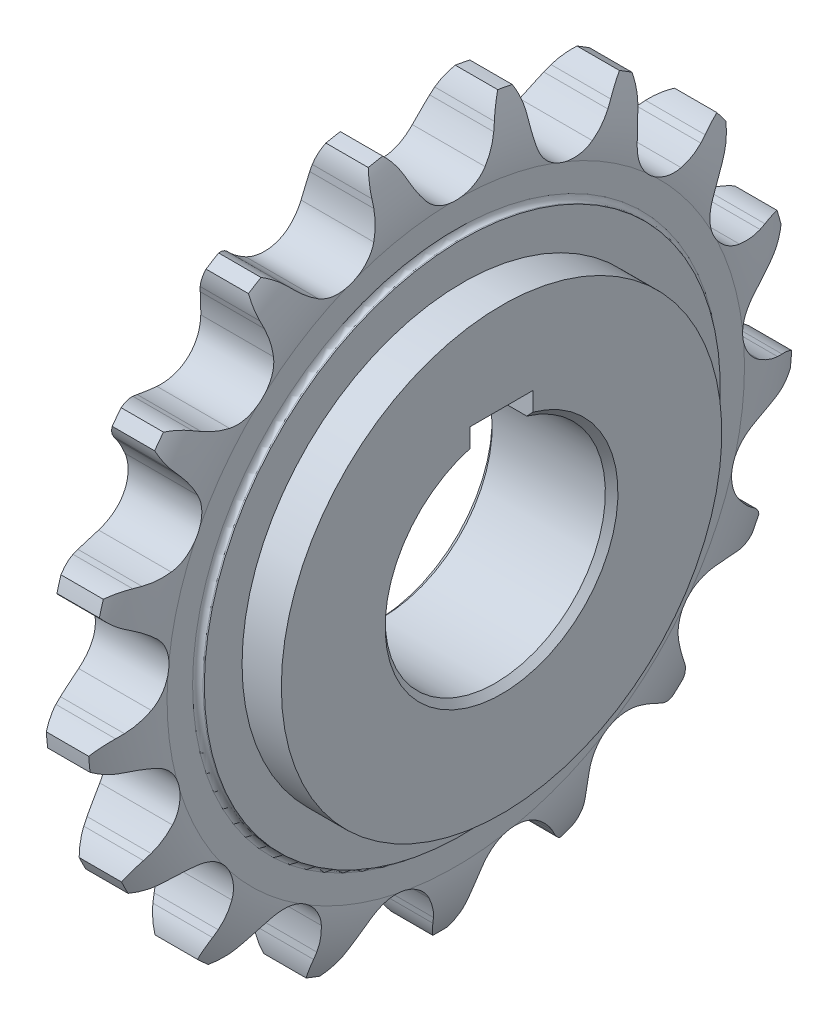
SolidWorks part; units mm, degrees
ref_plane "前视基准面" through (0, 0, 0) normal (0, 0, 1) x (1, 0, 0)
ref_plane "上视基准面" through (0, 0, 0) normal (0, 1, 0) x (1, 0, 0)
ref_plane "右视基准面" through (0, 0, 0) normal (1, 0, 0) x (0, 0, -1)
sketch "草图1" plane through (0, 0, 0) normal (0, 0, 1) x (1, 0, 0)
  line L0 (-9.525, 0) -> (9.525, 0) construction
  line L1 (-6.88, 17.5) -> (-6.88, 41)
  line L2 (-6.88, 41) -> (-6.673, 41)
  line L3 (-5.845, 41.8279) -> (-5.845, 45.8819)
  line L4 (-3.3685, 56) -> (3.3685, 56)
  line L5 (5.845, 45.8819) -> (5.845, 41.8279)
  line L6 (6.673, 41) -> (6.88, 41)
  line L7 (6.88, 41) -> (6.88, 17.5)
  line L8 (6.88, 17.5) -> (-6.88, 17.5)
  line L9 (0, 0) -> (0, 56) construction
  line L10 (-5.1196, 51.8369) -> (5.1196, 51.8369) construction
  line L11 (-5.1196, -51.8369) -> (5.1196, -51.8369) construction
  line L12 (9.525, 0) -> (26.525, 0) construction
  line L13 (-5.845, 45.8819) -> (3.7984, 45.8819) construction
  line L14 (-5.845, -45.8819) -> (3.7984, -45.8819) construction
  line L15 (26.525, 0) -> (38.435, 0) construction
  line L16 (38.435, 0) -> (56.515, 0) construction
  line L17 (56.515, 0) -> (69.085, 0) construction
  line L18 (69.085, 0) -> (91.865, 0) construction
  arc A0 (-3.3685, 56) -> (-5.845, 45.8819) centre (13.192, 46.5845) ccw
  arc A1 (3.3685, 56) -> (5.845, 45.8819) centre (-13.192, 46.5845) cw
  arc A2 (5.845, 41.8279) -> (6.673, 41) centre (6.673, 41.8279) ccw
  arc A3 (-6.673, 41) -> (-5.845, 41.8279) centre (-6.673, 41.8279) ccw
  point P30 (5.845, 41)
  point P33 (-5.845, 41)
  dimension "D1" = 4.8819
  dimension "rx" = 19.05
  dimension "D3" = 0.8279
  dimension "d" = 103.6737
  dimension "p" = 19.05
  dimension "z" = 17
  dimension "da" = 112
  dimension "df" = 91.7637
  dimension "dr" = 11.91
  dimension "dk" = 35
  dimension "dg" = 82
  dimension "h" = 18.08
  dimension "bf1" = 11.6901
  dimension "b1" = 12.57
  dimension "ba" = 2.4765
  dimension "D2" = 1.0349
  dimension "pt" = 22.78
revolve "旋转1" add sketch "草图1" angle 360 about L0
sketch "草图2" plane through (0, 0, 0) normal (1, 0, 0) x (0, 0, -1)
  line L0 (0, 0) -> (0, 56) construction
  line L1 (0, 0) -> (-10.29, 55.0465) construction
  line L2 (0, 0) -> (-20.2295, 52.2184) construction
  line L3 (4.7209, 48.0777) -> (9.6837, 44.126) construction
  line L4 (6.7831, 51.4859) -> (-7.4536, 57.772) construction
  line L5 (0, 0) -> (10.29, 55.0465) construction
  line L6 (6.7831, 51.4859) -> (7.2379, 52.516)
  line L7 (-6.7831, 51.4859) -> (-7.2379, 52.516)
  circle A0 centre (0, 0) radius 56 construction
  arc A1 (4.7209, 48.0777) -> (-4.7209, 48.0777) centre (0, 51.8369) cw
  arc A2 (4.7209, 48.0777) -> (6.7831, 51.4859) centre (-7.4536, 57.772) ccw
  arc A3 (9.1392, 55.2492) -> (7.2379, 52.516) centre (15.2194, 48.9919) ccw
  arc A4 (-4.7209, 48.0777) -> (-6.7831, 51.4859) centre (7.4536, 57.772) cw
  arc A5 (-9.1392, 55.2492) -> (-7.2379, 52.516) centre (-15.2194, 48.9919) cw
  arc A7 (9.1392, 55.2492) -> (-9.1392, 55.2492) centre (0, 0) ccw
  dimension "r1" = 6.0348
  dimension "r3" = 8.7248
  dimension "D1" = 21.176
  dimension "D2" = 10.588
  dimension "α/2" = 51.471
  dimension "M" = 7.4536
  dimension "T" = 5.9351
  dimension "β" = 14.706
  dimension "γ/2" = 13.235
  dimension "bc" = 1.1261
extrude "切除-拉伸1" cut sketch "草图2" against normal mid plane 13.7599
pattern_circular "阵列(圆周)1" count 17 over 360 about axis through (0, 0, 0) along (1, 0, 0) of "切除-拉伸1"
sketch "草图3" plane through (0, 0, 0) normal (0, 0, 1) x (1, 0, 0)
  line L0 (6.88, 17.5) -> (8.12, 17.5)
  line L3 (8.12, 17.5) -> (8.12, 30.7701)
  line L4 (8.12, 30.7701) -> (6.88, 30.7701)
  line L5 (6.88, 30.7701) -> (6.88, 17.5)
  line L6 (0, 0) -> (6.4, 0) construction
  line L8 (-6.88, 41) -> (-6.88, -41) construction
  dimension "h" = 13.2701
  dimension "K" = 6.4
  dimension "L" = 15
revolve "旋转2" [suppressed] add sketch "草图3" angle 360 about L6
sketch "草图4" plane through (-6.88, 0, 0) normal (-1, 0, 0) x (0, 0, 1)
  line L1 (-5, 16.7705) -> (5, 16.7705)
  line L2 (-5, 16.7705) -> (-5, 20.8)
  line L3 (-5, 20.8) -> (5, 20.8)
  line L4 (5, 16.7705) -> (5, 20.8)
  circle A0 centre (0, 0) radius 17.5 construction
  point P6 (1.7, 20.8)
  dimension "D1" = 20.8
  dimension "键槽宽度" = 10
  dimension "t1" = 3.3
extrude "切除-拉伸2" cut sketch "草图4" against normal through all
chamfer "倒角1" distance 1 angle 45 1 edges at (-6.88, -17.5, 0)
chamfer "倒角3" [suppressed] distance 1 angle 45
sketch "草图5" plane through (6.88, 0, 0) normal (1, 0, 0) x (0, 0, -1)
  line L1 (-5, 20.8) -> (5, 20.8)
  line L2 (-5, 20.8) -> (-5, 16.7705)
  line L4 (5, 20.8) -> (5, 16.7705)
  arc A0 (-5, 16.7705) -> (5, 16.7705) centre (0, 0) ccw
  circle A1 centre (0, 0) radius 35
extrude "凸台-拉伸1" add sketch "草图5" along normal blind 6.24
chamfer "倒角4" distance 1 angle 45 1 edges at (13.12, -17.5, 0)
